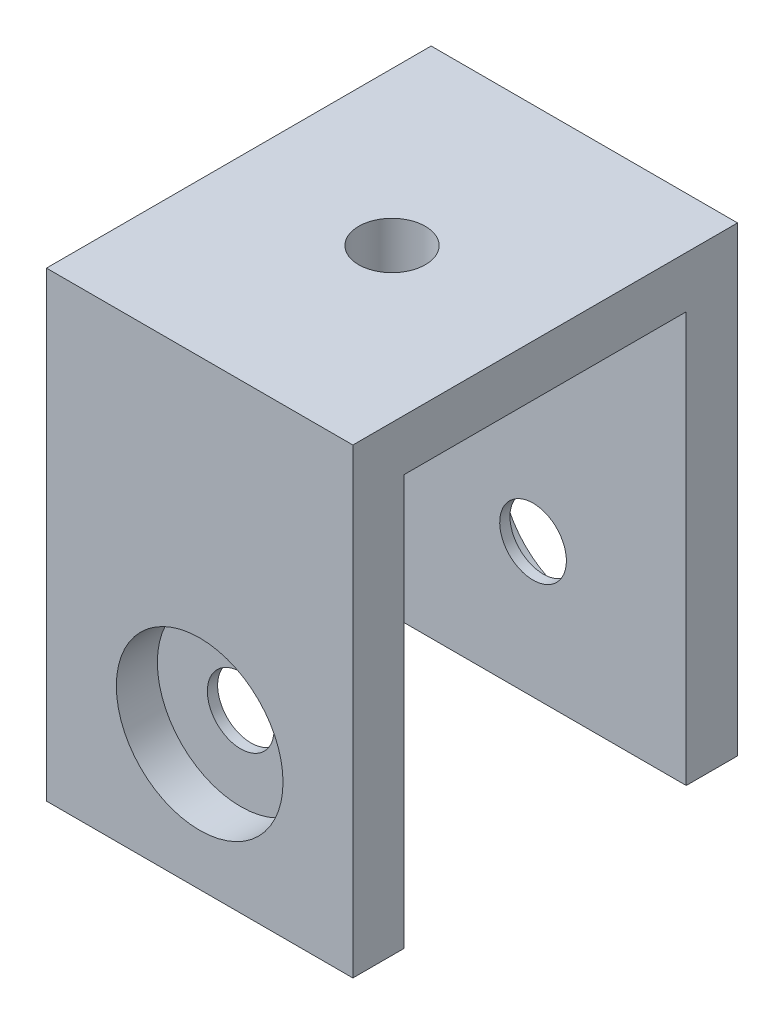
SolidWorks part; units mm, degrees
ref_plane "Front Plane" through (0, 0, 0) normal (0, 0, 1) x (1, 0, 0)
ref_plane "Top Plane" through (0, 0, 0) normal (0, 1, 0) x (1, 0, 0)
ref_plane "Right Plane" through (0, 0, 0) normal (1, 0, 0) x (0, 0, -1)
other "Configuration Table"
sketch "Sketch1" plane through (0, 0, 0) normal (0, 0, 1) x (1, 0, 0)
  line L1 (-11.9483, 12.75) -> (11.9483, 12.75)
  line L2 (-11.9483, 12.75) -> (-11.9483, -12.75)
  line L3 (-11.9483, -12.75) -> (11.9483, -12.75)
  line L4 (11.9483, 12.75) -> (11.9483, -12.75)
  line L5 (0, -12.75) -> (0, 12.75) construction
  line L6 (-11.9483, 0) -> (11.9483, 0) construction
  point P0 (0, 0)
  dimension "D1" = 25.5
extrude "Boss-Extrude1" add sketch "Sketch1" along normal blind 30
sketch "Sketch2" plane through (11.9483, 0, 0) normal (1, 0, 0) x (0, 0, -1)
  line L0 (-15, 12.75) -> (-15, -15.3237) construction
  line L1 (-30, 12.75) -> (0, 12.75) construction
  line L2 (-15, -12.75) -> (-20, -12.75)
  line L3 (-30, -12.75) -> (0, -12.75) construction
  line L4 (-15, -12.75) -> (-10, -12.75)
  line L5 (-20, -12.75) -> (-20, 2.25)
  line L6 (-20, 2.25) -> (-10, 2.25)
  line L7 (-10, 2.25) -> (-10, -12.75)
  dimension "D1" = 5
  dimension "D2" = 5
  dimension "D3" = 15
extrude "Cut-Extrude1" cut sketch "Sketch2" against normal through all
sketch "Sketch4" plane through (11.9483, 0, 0) normal (1, 0, 0) x (0, 0, -1)
  line L0 (-15, 12.75) -> (-15, -17.726) construction
  line L1 (-30, 12.75) -> (0, 12.75) construction
  line L2 (-10, 2.25) -> (-20, 2.25) construction
  line L3 (-10, 2.25) -> (-20, 2.25)
  line L4 (-20, 2.25) -> (-20, 7.25)
  line L5 (-20, 7.25) -> (-10, 7.25)
  line L6 (-10, 7.25) -> (-10, 2.25)
  dimension "D1" = 5
extrude "Cut-Extrude3" cut sketch "Sketch4" against normal through all
sketch "Sketch7" plane through (-11.9483, 0, 0) normal (-1, 0, 0) x (0, 0, 1)
  line L0 (10, -12.75) -> (4, -12.75)
  line L1 (10, -12.75) -> (0, -12.75) construction
  line L3 (20, 7.25) -> (26, 7.25)
  line L4 (10, 7.25) -> (10, -12.75)
  line L5 (10, 7.25) -> (4, 7.25)
  line L6 (4, 7.25) -> (4, -12.75)
  line L7 (15, 7.25) -> (15, -17.8195) construction
  line L8 (10, 7.25) -> (20, 7.25) construction
  line L9 (20, 7.25) -> (20, -12.75)
  line L10 (20, -12.75) -> (26, -12.75)
  line L11 (26, 7.25) -> (26, -12.75)
  dimension "D1" = 6
extrude "Cut-Extrude4" cut sketch "Sketch7" against normal up to surface (23.8966 mm away) up to face at (11.9483, -1.375, 15)
sketch "Sketch9" plane through (0, 12.75, 0) normal (0, 1, 0) x (1, 0, 0)
  line L4 (11.9483, 0) -> (-11.9483, 0)
  line L5 (11.9483, 0) -> (-11.9483, 0)
  line L6 (-11.9483, 0) -> (-11.9483, -30)
  line L7 (-11.9483, 0) -> (-11.9483, -30)
  line L8 (-11.9483, -30) -> (11.9483, -30)
  line L9 (-11.9483, -30) -> (11.9483, -30)
  line L10 (11.9483, -30) -> (11.9483, 0)
  line L11 (11.9483, -30) -> (11.9483, 0)
  dimension "D1" = 0
extrude "Boss-Extrude3" add sketch "Sketch9" along normal blind 17.5
sketch "Sketch12" plane through (0, 30.25, 0) normal (0, 1, 0) x (1, 0, 0)
  line L4 (11.9483, -30) -> (11.9483, 0)
  line L5 (11.9483, -30) -> (11.9483, 0)
  line L6 (11.9483, 0) -> (-11.9483, 0)
  line L7 (11.9483, 0) -> (-11.9483, 0)
  line L8 (-11.9483, 0) -> (-11.9483, -30)
  line L9 (-11.9483, 0) -> (-11.9483, -30)
  line L10 (-11.9483, -30) -> (11.9483, -30)
  line L11 (-11.9483, -30) -> (11.9483, -30)
  dimension "D1" = 0
extrude "Cut-Extrude7" cut sketch "Sketch12" against normal blind 8
sketch "Sketch15" plane through (0, 22.25, 0) normal (0, 1, 0) x (1, 0, 0)
  line L4 (-11.9483, -30) -> (11.9483, -30)
  line L5 (-11.9483, -30) -> (11.9483, -30)
  line L6 (11.9483, -30) -> (11.9483, 0)
  line L7 (11.9483, -30) -> (11.9483, 0)
  line L8 (11.9483, 0) -> (-11.9483, 0)
  line L9 (11.9483, 0) -> (-11.9483, 0)
  line L10 (-11.9483, 0) -> (-11.9483, -30)
  line L11 (-11.9483, 0) -> (-11.9483, -30)
  dimension "D1" = 0
extrude "Cut-Extrude11" cut sketch "Sketch15" against normal blind 6
sketch "Sketch18" plane through (0, -12.75, 0) normal (0, -1, 0) x (1, 0, 0)
  line L0 (-11.9483, 30) -> (-11.9483, 26) construction
  line L1 (-11.9483, 26) -> (11.9483, 26) construction
  line L2 (11.9483, 26) -> (11.9483, 30) construction
  line L3 (11.9483, 30) -> (-11.9483, 30) construction
  line L4 (11.9483, 0) -> (11.9483, 4) construction
  line L5 (11.9483, 4) -> (-11.9483, 4) construction
  line L6 (-11.9483, 4) -> (-11.9483, 0) construction
  line L7 (-11.9483, 0) -> (11.9483, 0) construction
  line L8 (-11.9483, 30) -> (-11.9483, 26)
  line L9 (-11.9483, 26) -> (11.9483, 26)
  line L10 (11.9483, 26) -> (11.9483, 30)
  line L11 (11.9483, 30) -> (-11.9483, 30)
  line L12 (11.9483, 0) -> (11.9483, 4)
  line L13 (11.9483, 4) -> (-11.9483, 4)
  line L14 (-11.9483, 4) -> (-11.9483, 0)
  line L15 (-11.9483, 0) -> (11.9483, 0)
extrude "Boss-Extrude4" add sketch "Sketch18" along normal blind 7
sketch "Sketch19" plane through (11.9483, 0, 0) normal (1, 0, 0) x (0, 0, -1)
  line L0 (0, -19.75) -> (0, 16.25) construction
  line L1 (-30, 16.25) -> (0, 16.25)
  line L2 (-30, 16.25) -> (-30, 11.25)
  line L3 (-30, 11.25) -> (0, 11.25)
  line L4 (0, 16.25) -> (0, 11.25)
  line L5 (-4, 7.25) -> (-26, 7.25) construction
  dimension "D1" = 4
extrude "Cut-Extrude12" cut sketch "Sketch19" against normal through all
sketch "Sketch20" plane through (0, 11.25, 0) normal (0, 1, 0) x (1, 0, 0)
  line L0 (-11.9483, 0) -> (11.9483, -30) construction
  line L1 (11.9483, 0) -> (-11.9483, -30) construction
  line L2 (-11.9483, -30) -> (-11.9483, 0) construction
  circle A0 centre (0, -15) radius 2.6
  dimension "D1" = 5.2
extrude "Cut-Extrude13" cut sketch "Sketch20" against normal through all
sketch "Sketch21" plane through (0, -19.75, 0) normal (0, -1, 0) x (1, 0, 0)
  line L0 (-11.9483, 0) -> (11.9483, 0) construction
  line L1 (11.9483, 0) -> (11.9483, 4) construction
  line L2 (11.9483, 4) -> (-11.9483, 4) construction
  line L3 (-11.9483, 4) -> (-11.9483, 0) construction
  line L4 (11.9483, 30) -> (-11.9483, 30) construction
  line L5 (-11.9483, 30) -> (-11.9483, 26) construction
  line L6 (-11.9483, 26) -> (11.9483, 26) construction
  line L7 (11.9483, 26) -> (11.9483, 30) construction
  line L8 (-11.9483, 0) -> (11.9483, 0)
  line L9 (11.9483, 0) -> (11.9483, 4)
  line L10 (11.9483, 4) -> (-11.9483, 4)
  line L11 (-11.9483, 4) -> (-11.9483, 0)
  line L12 (11.9483, 30) -> (-11.9483, 30)
  line L13 (-11.9483, 30) -> (-11.9483, 26)
  line L14 (-11.9483, 26) -> (11.9483, 26)
  line L15 (11.9483, 26) -> (11.9483, 30)
extrude "Boss-Extrude5" add sketch "Sketch21" along normal blind 5
sketch "Sketch22" plane through (0, 0, 30) normal (0, 0, 1) x (1, 0, 0)
  line L0 (0, 11.25) -> (0, -24.75) construction
  line L1 (-11.9483, 11.25) -> (11.9483, 11.25) construction
  line L2 (11.9483, -24.75) -> (-11.9483, -24.75) construction
  circle A0 centre (0, -14.25) radius 2.6
  dimension "D1" = 5.2
  dimension "D2" = 10.5
extrude "Cut-Extrude14" cut sketch "Sketch22" against normal through all
sketch "Sketch23" plane through (0, 0, 0) normal (0, 0, -1) x (-1, 0, 0)
  circle A0 centre (0, -14.25) radius 6.5
  dimension "D1" = 13
extrude "Cut-Extrude15" cut sketch "Sketch23" against normal blind 3.2
ref_plane "Plane1" through (0, 0, 15) normal (0, 0, -1) x (-1, 0, 0)
mirror "Mirror1" about plane through (0, 0, 15) normal (0, 0, -1) of "Cut-Extrude15"
